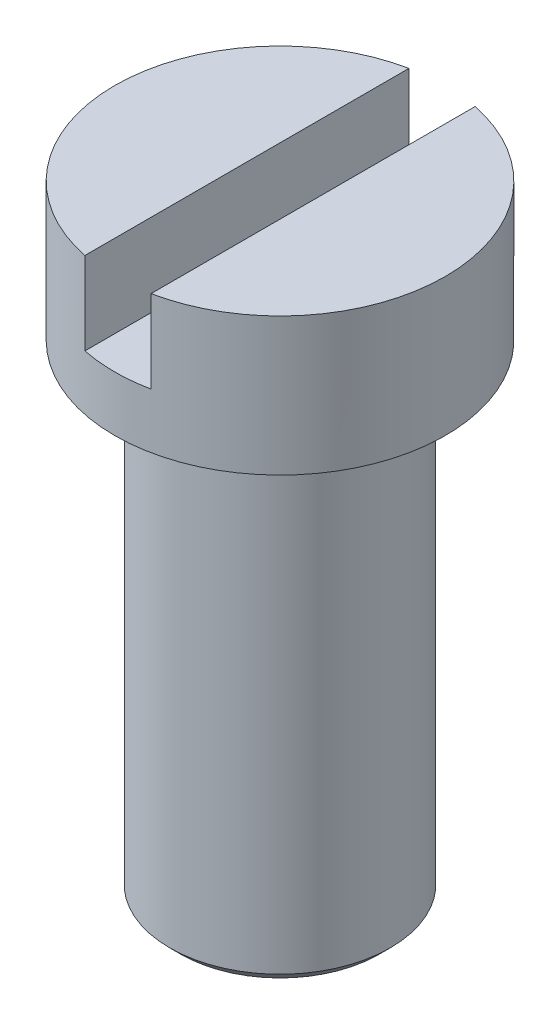
from build123d import *

# Parameters (mm, degrees)
SKETCH_1_R          = 20
EXTRUDE_1_DEPTH     = 50
SKETCH_2_R          = 30
EXTRUDE_2_DEPTH     = 12.5
CHAMFER_1_SIZE      = 2
SKETCH_3_W          = 12
SKETCH_3_H          = 77.498414616
CUT_EXTRUDE_1_DEPTH = 15


with BuildPart() as part:
    # 草图1 → 凸台-拉伸1 (new, symmetric)
    with BuildSketch(Plane(origin=(0, 0, 0), x_dir=(1, 0, 0), z_dir=(0, 1, 0))):
        with Locations(Location((0, 0, 0), (0, 0, 270))):
            Circle(SKETCH_1_R)
    extrude(amount=EXTRUDE_1_DEPTH, both=True)

    # 草图2 → 凸台-拉伸2 (add, symmetric)
    with BuildSketch(Plane(origin=(0, 50, 0), x_dir=(1, 0, 0), z_dir=(0, 1, 0))):
        with Locations(Location((0, 0, 0), (0, 0, 270))):
            Circle(SKETCH_2_R)
    extrude(amount=EXTRUDE_2_DEPTH, both=True)

    # 倒角1
    chamfer_1_edges = [part.edges().sort_by_distance(p)[0] for p in [
        (0, -50, -20),
    ]]
    chamfer(chamfer_1_edges, length=CHAMFER_1_SIZE)

    # 草图3 → 切除-拉伸1 (cut)
    with BuildSketch(Plane(origin=(0, 62.5, 0), x_dir=(1, 0, 0), z_dir=(0, 1, 0))):
        Rectangle(SKETCH_3_W, SKETCH_3_H)
    extrude(amount=-CUT_EXTRUDE_1_DEPTH, mode=Mode.SUBTRACT)


solid = part.part
